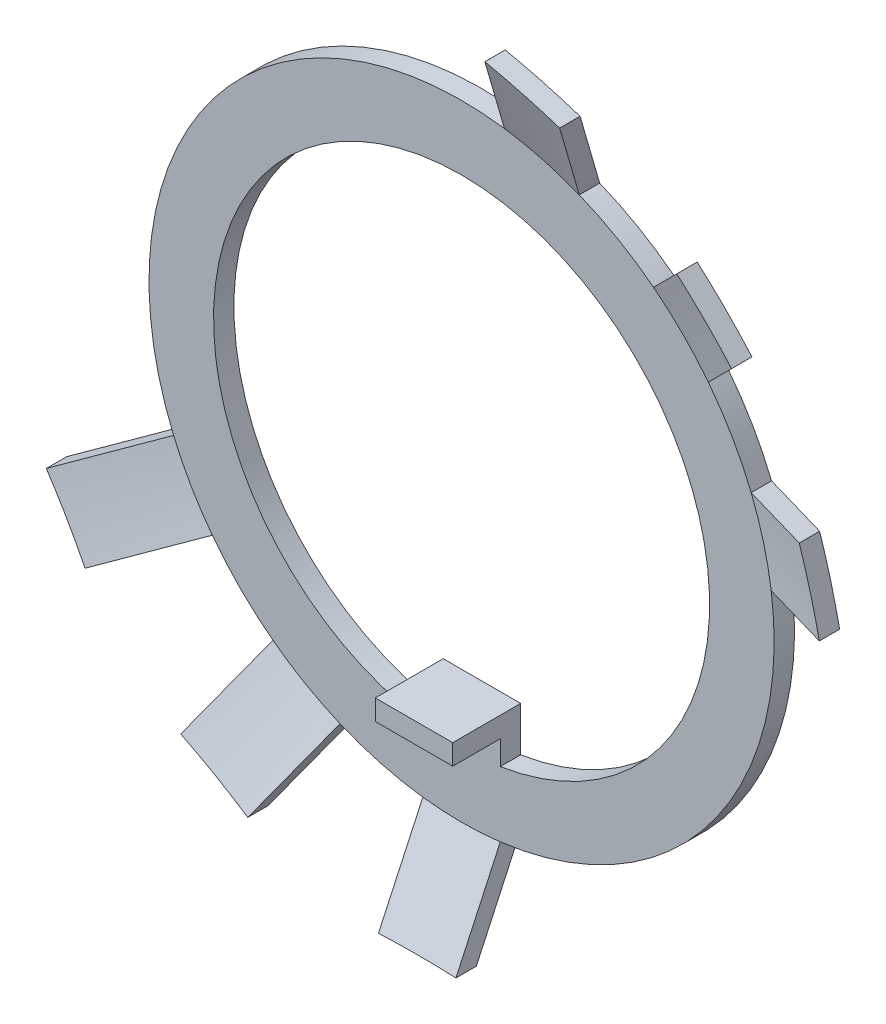
SolidWorks part; units mm, degrees
ref_plane "前视" through (0, 0, 0) normal (0, 0, 1) x (1, 0, 0)
ref_plane "上视" through (0, 0, 0) normal (0, 1, 0) x (1, 0, 0)
ref_plane "右视" through (0, 0, 0) normal (1, 0, 0) x (0, 0, -1)
sketch "尺寸草图" plane through (0, 0, 0) normal (0, 0, 1) x (1, 0, 0)
  line L0 (0, 0) -> (30, 0) construction
  line L1 (0, 0) -> (0, -30) construction
  circle A0 centre (0, 0) radius 30 construction
  point P5 (7.2, 0)
  point P6 (25, 0)
  point P7 (5.7, 0)
  point P8 (-3, 0)
  point P10 (-6.5, 0)
  point P12 (0, 16)
  dimension "D1" = 46
  dimension "DD" = 60
  dimension "a" = 33
  dimension "b" = 5.7
  dimension "h" = 5
  dimension "s" = 1.5
  dimension "d" = 36.5
sketch "草图2" plane through (0, 0, 0) normal (1, 0, 0) x (0, 0, -1)
  line L0 (0, 0) -> (-1.5, 0) construction
  line L1 (-3.2642, 30) -> (0, 23)
  line L2 (0, 23) -> (0, 0)
  line L3 (-3.2642, 30) -> (-4.7642, 30)
  line L4 (-4.7642, 30) -> (-1.5, 23)
  line L5 (-1.5, 23) -> (-1.5, 0)
  line L6 (0, 0) -> (-1.5, 0)
  dimension "D1" = 1.5
  dimension "D2" = 155
  dimension "D3" = 46
  dimension "D4" = 60
revolve "基体-旋转" add sketch "草图2" angle 360 about L0
sketch "草图3" plane through (0, 0, 0) normal (0, 0, 1) x (1, 0, 0)
  line L0 (0, 0) -> (0, -29.8643) construction
  line L1 (-2.85, -22.8227) -> (-2.85, -29.8643)
  line L2 (-2.85, -29.8643) -> (2.85, -29.8643)
  line L3 (2.85, -22.8227) -> (2.85, -29.8643)
  line L4 (2.85, -18.0261) -> (2.85, -14.75)
  line L5 (2.85, -14.75) -> (-2.85, -14.75)
  line L6 (-2.85, -18.0261) -> (-2.85, -14.75)
  line L7 (0, 0) -> (-14.9322, -25.8633) construction
  line L8 (0, 0) -> (-25.8633, -14.9322) construction
  line L9 (0, 0) -> (28.8467, 7.7295) construction
  line L10 (0, 0) -> (21.1173, 21.1173) construction
  line L11 (0, 0) -> (7.7295, 28.8467) construction
  line L12 (0, 0) -> (30, 0) construction
  line L13 (-17.4003, -24.4383) -> (-12.464, -27.2883)
  line L14 (-12.464, -27.2883) -> (-8.9432, -21.1901)
  line L15 (-17.4003, -24.4383) -> (-13.8795, -18.3401)
  line L16 (-18.3401, -13.8795) -> (-24.4383, -17.4003)
  line L17 (-24.4383, -17.4003) -> (-27.2883, -12.464)
  line L18 (-21.1901, -8.9432) -> (-27.2883, -12.464)
  line L19 (4.9766, 29.5844) -> (10.4823, 28.1091)
  line L20 (10.4823, 28.1091) -> (8.6598, 21.3074)
  line L21 (4.9766, 29.5844) -> (3.1541, 22.7827)
  line L22 (14.1229, 18.1534) -> (19.102, 23.1325)
  line L23 (19.102, 23.1325) -> (23.1325, 19.102)
  line L24 (18.1534, 14.1229) -> (23.1325, 19.102)
  line L25 (21.3074, 8.6598) -> (28.1091, 10.4823)
  line L26 (28.1091, 10.4823) -> (29.5844, 4.9766)
  line L27 (22.7827, 3.1541) -> (29.5844, 4.9766)
  arc A0 (2.85, -18.0261) -> (-2.85, -18.0261) centre (0, 0) ccw
  arc A1 (2.85, -22.8227) -> (22.7827, 3.1541) centre (0, 0) ccw
  circle A3 centre (0, 0) radius 30 construction
  arc A4 (-8.9432, -21.1901) -> (-2.85, -22.8227) centre (0, 0) ccw
  arc A5 (-18.3401, -13.8795) -> (-13.8795, -18.3401) centre (0, 0) ccw
  arc A6 (21.3074, 8.6598) -> (18.1534, 14.1229) centre (0, 0) ccw
  arc A7 (14.1229, 18.1534) -> (8.6598, 21.3074) centre (0, 0) ccw
  arc A8 (3.1541, 22.7827) -> (-21.1901, -8.9432) centre (0, 0) ccw
  point P14 (0, -14.75)
  point P25 (-14.9322, -25.8633)
  point P31 (-25.8633, -14.9322)
  point P35 (7.7295, 28.8467)
  point P40 (21.1173, 21.1173)
  point P45 (28.8467, 7.7295)
  dimension "D1" = 46
  dimension "D2" = 36.5
  dimension "D4" = 33
  dimension "D7" = 15
extrude "切除-拉伸2" cut sketch "草图3" along normal up to next flip side to cut
sketch "草图4" plane through (0, 0, 0) normal (0, 0, 1) x (1, 0, 0)
  line L0 (2.85, -14.75) -> (2.85, -18.0261) construction
  line L1 (-2.85, -14.75) -> (2.85, -14.75)
  line L2 (-2.85, -14.75) -> (-2.85, -16.25)
  line L3 (-2.85, -16.25) -> (2.85, -16.25)
  line L4 (2.85, -14.75) -> (2.85, -16.25)
  dimension "D1" = 1.5
extrude "凸台-拉伸1" add sketch "草图4" along normal blind 5
